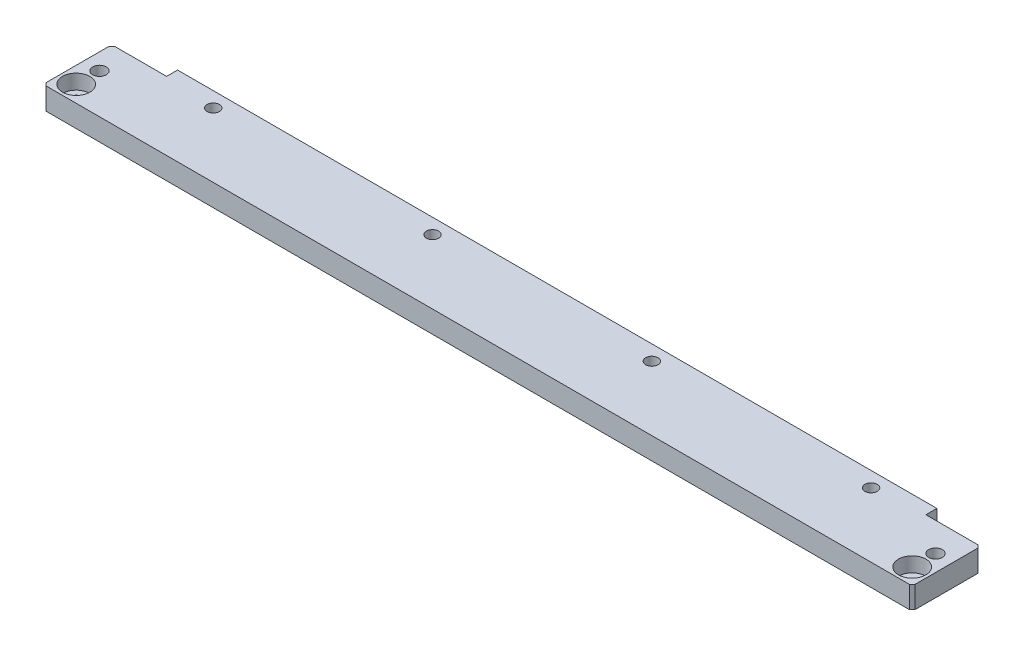
from build123d import *

# Parameters (mm, degrees)
SKETCH_1_W                   = 317
SKETCH_1_H                   = 25
EXTRUDE_1_DEPTH              = 8
HOLE_WIZARD_M5_1_D           = 5.5
HOLE_WIZARD_M5_1_CBORE_D     = 10
HOLE_WIZARD_M5_1_CBORE_DEPTH = 5.4
SKETCH_4_R                   = 2.5
CUT_EXTRUDE_1_DEPTH          = 160.193278753
SKETCH_7_W                   = 277
SKETCH_7_H                   = 4
EXTRUDE_2_DEPTH              = 8
HOLE_WIZARD_M4_1_D           = 4.5
HOLE_WIZARD_M4_1_CBORE_D     = 8
HOLE_WIZARD_M4_1_CBORE_DEPTH = 4.4
CHAMFER_3_SIZE               = 1


with BuildPart() as part:
    # 草图1 → 凸台-拉伸1 (new body)
    with BuildSketch(Plane(origin=(0, 0, 0), x_dir=(1, 0, 0), z_dir=(0, 1, 0))):
        Rectangle(SKETCH_1_W, SKETCH_1_H)
    extrude(amount=EXTRUDE_1_DEPTH)

    # M5 六角凹头螺钉的柱形沉头孔1 (through all)
    with Locations(Plane(origin=(0, 8, 0), x_dir=(1, 0, 0), z_dir=(0, 1, 0))):
        with Locations((-152.5, -6.5), (152.5, -6.5)):
            CounterBoreHole(HOLE_WIZARD_M5_1_D / 2, HOLE_WIZARD_M5_1_CBORE_D / 2, HOLE_WIZARD_M5_1_CBORE_DEPTH)

    # 草图4 → 切除-拉伸1 (cut, through all)
    with BuildSketch(Plane(origin=(0, 8, 0), x_dir=(1, 0, 0), z_dir=(0, 1, 0))):
        with Locations(Location((-152.5, 2, 0), (0, 0, 270))):
            Circle(SKETCH_4_R)
        with Locations(Location((152.5, 2, 0), (0, 0, 270))):
            Circle(SKETCH_4_R)
    extrude(amount=-CUT_EXTRUDE_1_DEPTH, mode=Mode.SUBTRACT)

    # 草图7 → 凸台-拉伸2 (add)
    with BuildSketch(Plane.XZ):
        with Locations((0, -14.5)):
            Rectangle(SKETCH_7_W, SKETCH_7_H)
    extrude(amount=-EXTRUDE_2_DEPTH)

    # M4 六角凹头螺钉的柱形沉头孔1 (through all)
    with Locations(Plane(origin=(0, 0, 0), x_dir=(-1, 0, 0), z_dir=(0, -1, 0))):
        with Locations((-120, 11), (-40, 11), (40, 11), (120, 11)):
            CounterBoreHole(HOLE_WIZARD_M4_1_D / 2, HOLE_WIZARD_M4_1_CBORE_D / 2, HOLE_WIZARD_M4_1_CBORE_DEPTH)

    # 倒角3
    chamfer_3_edges = [part.edges().sort_by_distance(p)[0] for p in [
        (-158.5, 4, -12.5),
        (-158.5, 4, 12.5),
        (158.5, 4, -12.5),
        (158.5, 4, 12.5),
    ]]
    chamfer(chamfer_3_edges, length=CHAMFER_3_SIZE)


solid = part.part
